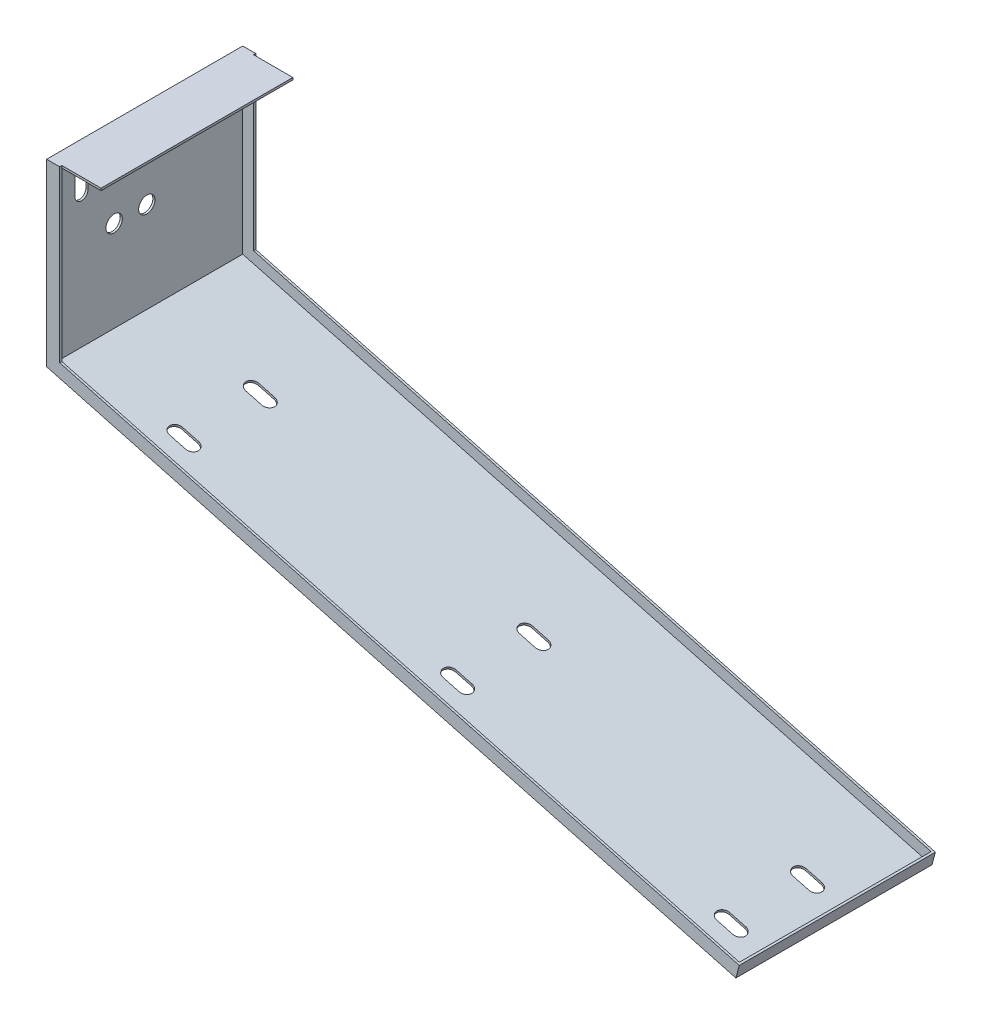
from build123d import *

# Parameters (mm, degrees)
EXTRUDE_THIN1_DEPTH  = 176
EXTRUDE_THIN2_DEPTH  = 2
EXTRUDE_THIN3_DEPTH  = 2
SKETCH4_W            = 2
SKETCH4_H            = 176
BOSS_EXTRUDE1_DEPTH  = 10
CUT_EXTRUDE1_DEPTH   = 2
CUT_EXTRUDE2_DEPTH   = 2
SKETCH7_R            = 7.5
CUT_EXTRUDE3_DEPTH   = 2
LPATTERN3_COUNT      = 2
LPATTERN3_PITCH      = 30
LPATTERN4_COUNT      = 2
LPATTERN4_PITCH      = 70
LPATTERN4_COUNT_DIR2 = 3
LPATTERN4_PITCH_DIR2 = 260
LPATTERN5_COUNT      = 2
LPATTERN5_PITCH      = 70


with BuildPart() as part:
    # Sketch1 → Extrude-Thin1 (new body)
    with BuildSketch(Plane.XY):
        Polygon((632.681416219, -169.526474542), (0, 0), (0, 165), (48, 165), (48, 163), (2, 163), (2, 1.534653976), (633.19905431, -167.59462289), align=None)
    extrude(amount=EXTRUDE_THIN1_DEPTH)

    # Sketch2 → Extrude-Thin2 (add)
    with BuildSketch(Plane.XY.offset(176)):
        Polygon((0, 165), (0, 0), (632.681416219, -169.526474542), (635.787244761, -157.935364627), (12, 9.207923856), (12, 165), align=None)
    extrude(amount=EXTRUDE_THIN2_DEPTH)

    # Sketch3 → Extrude-Thin3 (add)
    with BuildSketch(Plane(origin=(0, 0, 0), x_dir=(-1, 0, 0), z_dir=(0, 0, -1))):
        Polygon((0, 165), (0, 0), (-632.681416219, -169.526474542), (-635.787244761, -157.935364627), (-12, 9.207923856), (-12, 165), align=None)
    extrude(amount=EXTRUDE_THIN3_DEPTH)

    # Sketch4 → Boss-Extrude1 (add)
    with BuildSketch(Plane(origin=(0.51763809, 1.931851653, 0), x_dir=(0.9659258262890673, -0.25881904510252474, 0), z_dir=(0.25881904510252474, 0.9659258262890673, 0))):
        with Locations((654, -88)):
            Rectangle(SKETCH4_W, SKETCH4_H)
    extrude(amount=BOSS_EXTRUDE1_DEPTH)

    # Sketch5 → Cut-Extrude1 (cut)
    with BuildSketch(Plane(origin=(0, 0, 0), x_dir=(0.9659258262890673, -0.2588190451025247, 0), z_dir=(-0.2588190451025247, -0.9659258262890673, 0))):
        with BuildLine():
            Line((611.5, 154), (626.5, 154))
            ThreePointArc((626.5, 154), (632.5, 148), (626.5, 142))
            Line((626.5, 142), (611.5, 142))
            ThreePointArc((611.5, 142), (605.5, 148), (611.5, 154))
        make_face()
    cut_extrude1 = extrude(amount=-CUT_EXTRUDE1_DEPTH, mode=Mode.SUBTRACT)

    # Sketch6 → Cut-Extrude2 (cut)
    with BuildSketch(Plane(origin=(2, 0, 0), x_dir=(0, 0, -1), z_dir=(1, 0, 0))):
        with BuildLine():
            Line((-142, 139.034653976), (-142, 124.034653976))
            ThreePointArc((-142, 124.034653976), (-148, 118.034653976), (-154, 124.034653976))
            Line((-154, 124.034653976), (-154, 139.034653976))
            ThreePointArc((-154, 139.034653976), (-148, 145.034653976), (-142, 139.034653976))
        make_face()
    cut_extrude2 = extrude(amount=-CUT_EXTRUDE2_DEPTH, mode=Mode.SUBTRACT)

    # Sketch7 → Cut-Extrude3 (cut)
    with BuildSketch(Plane.ZY):
        with Locations((88, 85)):
            Circle(SKETCH7_R)
    cut_extrude3 = extrude(amount=-CUT_EXTRUDE3_DEPTH, mode=Mode.SUBTRACT)

    # LPattern3: Cut-Extrude3 ×2
    with Locations(*[(0, 0, i * LPATTERN3_PITCH) for i in range(1, LPATTERN3_COUNT)]):
        add(cut_extrude3, mode=Mode.SUBTRACT)

    # LPattern4: Cut-Extrude1 2 × 3
    with Locations(*[Vector(0, 0, -1) * (i * LPATTERN4_PITCH) + Vector(-0.9659258262890673, 0.2588190451025247, 0) * (j * LPATTERN4_PITCH_DIR2) for i in range(LPATTERN4_COUNT) for j in range(LPATTERN4_COUNT_DIR2) if (i, j) != (0, 0)]):
        add(cut_extrude1, mode=Mode.SUBTRACT)

    # LPattern5: Cut-Extrude2 ×2
    with Locations(*[(0, 0, -i * LPATTERN5_PITCH) for i in range(1, LPATTERN5_COUNT)]):
        add(cut_extrude2, mode=Mode.SUBTRACT)


solid = part.part
